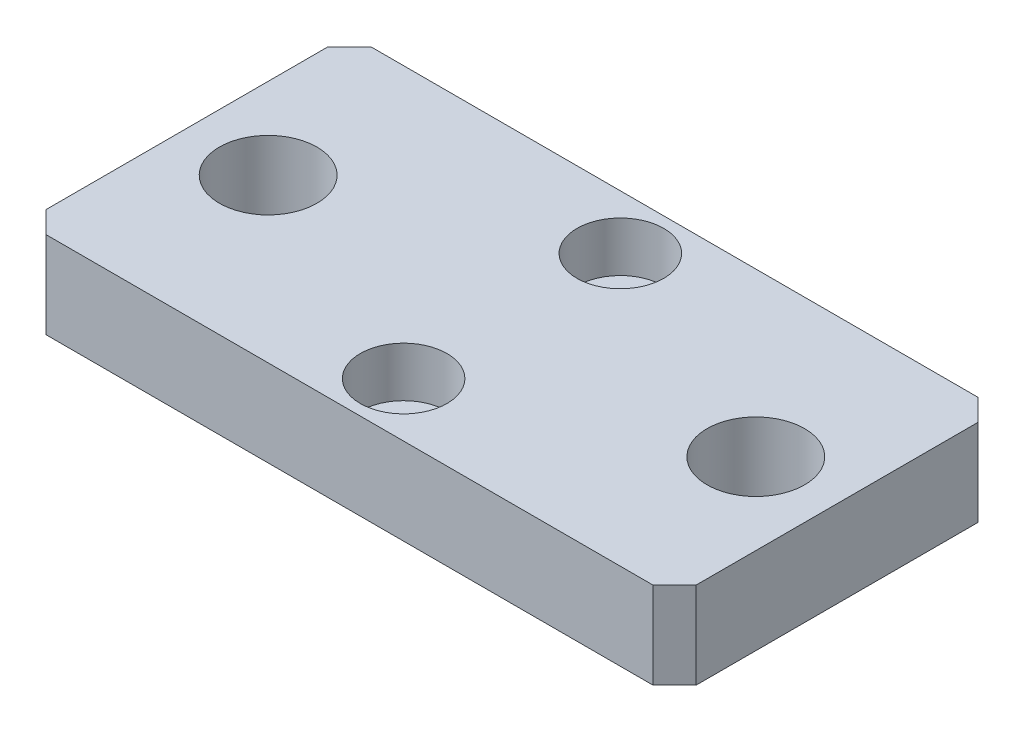
SolidWorks part; units mm, degrees
material "A6061"
ref_plane "前基準面" through (0, 0, 0) normal (0, 0, 1) x (1, 0, 0)
ref_plane "上基準面" through (0, 0, 0) normal (0, 1, 0) x (1, 0, 0)
ref_plane "右基準面" through (0, 0, 0) normal (1, 0, 0) x (0, 0, -1)
sketch "草图1" plane through (0, 0, 0) normal (0, 1, 0) x (1, 0, 0)
  line L1 (-30, -15) -> (30, -15)
  line L2 (-30, -15) -> (-30, 15)
  line L3 (-30, 15) -> (30, 15)
  line L4 (30, -15) -> (30, 15)
  line L5 (-30, -15) -> (30, 15) construction
  line L6 (-30, 15) -> (30, -15) construction
  point P0 (0, 0)
  dimension "D1" = 60
  dimension "D2" = 30
extrude "凸台-拉伸1" add sketch "草图1" along normal mid plane 8
chamfer "倒角1" distance 2 angle 45 4 edges at (-30, 0, 15) (-30, 0, -15) (30, 0, 15) (30, 0, -15)
hole_wizard "打孔尺寸(%根据)内六角圆柱头螺钉的类型1" positions "草图2" profile "草图3" counterbore size "M4" standard "GB" end condition through all
sketch "草图2" plane through (0, 4, 0) normal (0, 1, 0) x (1, 0, 0)
  line L0 (17.9144, 0) -> (0, 0) construction
  point P0 (0, -10)
  point P8 (0, 10)
  dimension "D1" = 20
sketch "草图3" plane through (0, 4, 10) normal (1, 0, 0) x (0, 0, 1)
  line L0 (0, 0) -> (0, 8)
  line L1 (0, 8) -> (2.25, 8)
  line L3 (2.25, 8) -> (2.25, 4.6)
  line L4 (2.25, 4.6) -> (4, 4.6)
  line L5 (4, 4.6) -> (4, 0)
  line L7 (4, 0) -> (0, 0)
  line L11 (0, -6.35) -> (0, 107.95) construction
  dimension "通孔孔直径" = 4.5
  dimension "通孔孔深度" = 8
  dimension "柱形沉头孔直径" = 8
  dimension "柱形沉头孔深度" = 4.6
hole_wizard "M10x1.0 螺纹孔1" positions "草图4" profile "草图5" tap size "M10x1.0" standard "GB" end condition through all
sketch "草图4" plane through (0, -4, 0) normal (0, -1, 0) x (-1, 0, 0)
  line L0 (0, 23.966) -> (0, 0) construction
  point P0 (-22.5, 0)
  point P7 (22.5, 0)
  dimension "D1" = 45
sketch "草图5" plane through (22.5, -4, 0) normal (1, 0, 0) x (0, 0, -1)
  line L0 (0, 0) -> (0, 8)
  line L1 (0, 8) -> (4.5, 8)
  line L2 (4.5, 8) -> (4.5, 0)
  line L5 (4.5, 0) -> (0, 0)
  line L11 (0, -6.35) -> (0, 107.95) construction
  dimension "通孔螺纹孔钻头直径" = 9
  dimension "通孔螺纹孔钻头深度" = 8
cosmetic thread "孔螺蚊线1"
cosmetic thread "孔螺蚊线2"
